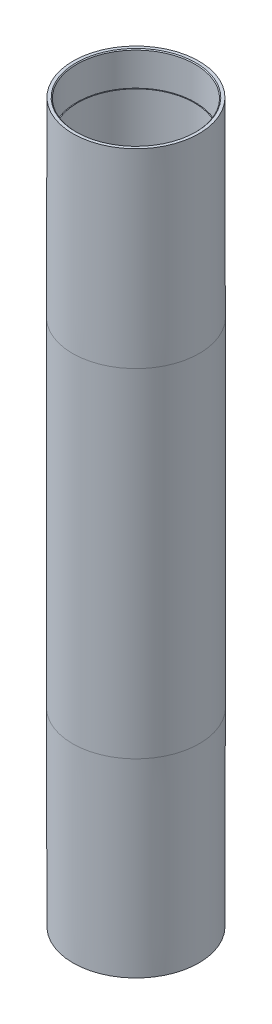
from build123d import *

# Parameters (mm, degrees)
SKETCH_2_R          = 70
CUT_EXTRUDE_1_DEPTH = 40
CUT_EXTRUDE_START   = -40
SKETCH_3_R          = 70
CUT_EXTRUDE_2_DEPTH = 40
SKETCH_4_R          = 69
CUT_EXTRUDE_3_DEPTH = 843
CHAMFER_1_SIZE      = 1


with BuildPart() as part:
    # 草图1 → 旋转1 (revolve)
    with BuildSketch(Plane.XY, mode=Mode.PRIVATE) as revolve_1_sk:
        Polygon((0, 0), (-0.5, 225), (-0.5, 625), (0, 850), (74.5, 850), (74.5, 0), align=None)
    revolve(revolve_1_sk.sketch.rotate(Axis((74.5, 850, 0), (0, -1, 0)), 270), axis=Axis((74.5, 850, 0), (0, -1, 0)))

    # 草图2 → 切除-拉伸1 (cut)
    with BuildSketch(Plane(origin=(0, 850, 0), x_dir=(1, 0, 0), z_dir=(0, 1, 0))):
        with Locations(Location((74.5, 0, 0), (0, 0, 270))):
            Circle(SKETCH_2_R)
    extrude(amount=-CUT_EXTRUDE_1_DEPTH, mode=Mode.SUBTRACT)

    # 草图3 → 切除-拉伸2 (cut)
    with BuildSketch(Plane.XZ.offset(CUT_EXTRUDE_START)):
        with Locations(Location((74.5, 0, 0), (0, 0, 90))):
            Circle(SKETCH_3_R)
    extrude(amount=CUT_EXTRUDE_2_DEPTH, mode=Mode.SUBTRACT)

    # 草图4 → 切除-拉伸3 (cut)
    with BuildSketch(Plane.XZ.offset(-40)):
        with Locations(Location((74.5, 0, 0), (0, 0, 270))):
            Circle(SKETCH_4_R)
    extrude(amount=-CUT_EXTRUDE_3_DEPTH, mode=Mode.SUBTRACT)

    # 倒角1
    chamfer_1_edges = [part.edges().sort_by_distance(p)[0] for p in [
        (74.5, 850, -70),
        (74.5, 0, -70),
    ]]
    chamfer(chamfer_1_edges, length=CHAMFER_1_SIZE)


solid = part.part
